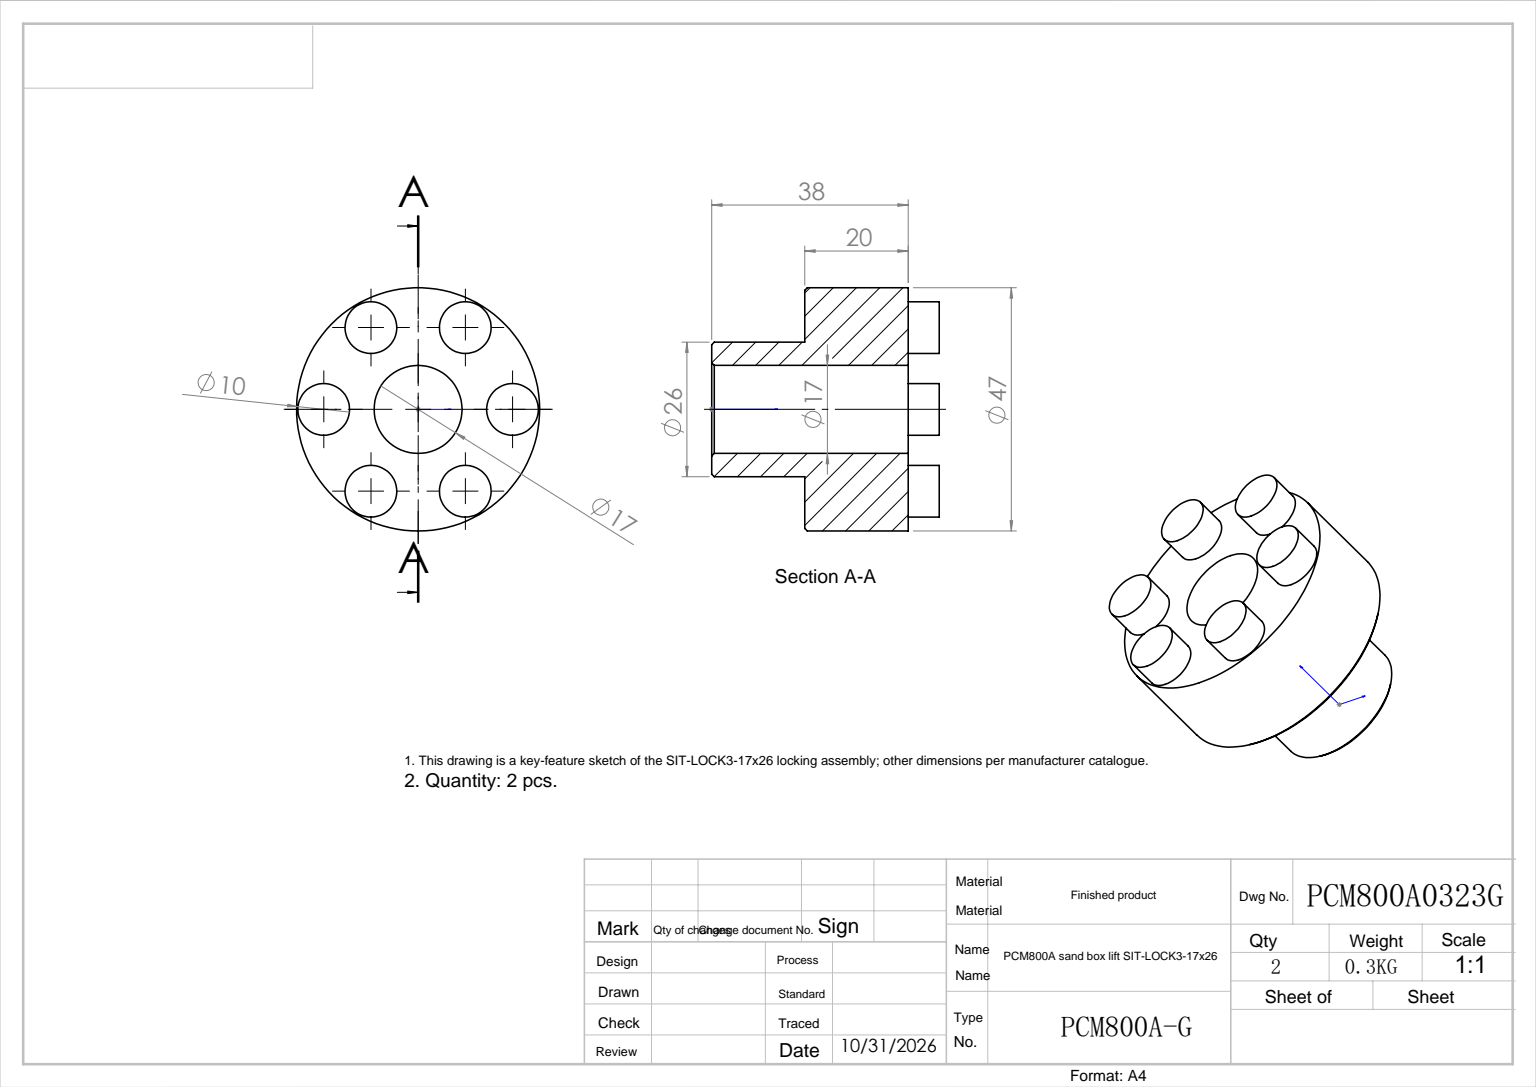
from build123d import *

# Parameters (mm, degrees)
SKETCH_1_R          = 13
SKETCH_1_R_2        = 8.5
EXTRUDE_1_DEPTH     = 18
SKETCH_2_R          = 23.5
EXTRUDE_2_DEPTH     = 20
SKETCH_3_R          = 8.5
CUT_EXTRUDE_1_DEPTH = 39.787884706
SKETCH_4_R          = 5
EXTRUDE_3_DEPTH     = 6
CHAMFER_1_SIZE      = 0.5


with BuildPart() as part:
    # 草图1 → 拉伸1 (new body)
    with BuildSketch(Plane(origin=(0, 0, 0), x_dir=(1, 0, 0), z_dir=(0, 1, 0))):
        with Locations(Location((0, 0, 0), (0, 0, 270))):
            Circle(SKETCH_1_R)
        with Locations(Location((0, 0, 0), (0, 0, 270))):
            Circle(SKETCH_1_R_2, mode=Mode.SUBTRACT)
    extrude(amount=EXTRUDE_1_DEPTH)

    # 草图2 → 拉伸2 (add)
    with BuildSketch(Plane(origin=(0, 18, 0), x_dir=(-1, 0, 0), z_dir=(0, 1, 0))):
        with Locations(Location((0, 0, 0), (0, 0, 90))):
            Circle(SKETCH_2_R)
    extrude(amount=EXTRUDE_2_DEPTH)

    # 草图3 → 切除-拉伸1 (cut, through all)
    with BuildSketch(Plane.XZ.offset(-18)):
        with Locations(Location((0, 0, 0), (0, 0, 270))):
            Circle(SKETCH_3_R)
    extrude(amount=-CUT_EXTRUDE_1_DEPTH, mode=Mode.SUBTRACT)

    # 草图4 → 拉伸3 (add)
    with BuildSketch(Plane(origin=(0, 38, 0), x_dir=(-1, 0, 0), z_dir=(0, 1, 0))):
        with Locations(Location((-18.25, 0, 0), (0, 0, 90))):
            Circle(SKETCH_4_R)
        with Locations(Location((-9.125, 15.804963619, 0), (0, 0, 90))):
            Circle(SKETCH_4_R)
        with Locations(Location((9.125, 15.804963619, 0), (0, 0, 90))):
            Circle(SKETCH_4_R)
        with Locations(Location((18.25, 0, 0), (0, 0, 90))):
            Circle(SKETCH_4_R)
        with Locations(Location((9.125, -15.804963619, 0), (0, 0, 90))):
            Circle(SKETCH_4_R)
        with Locations(Location((-9.125, -15.804963619, 0), (0, 0, 90))):
            Circle(SKETCH_4_R)
    extrude(amount=EXTRUDE_3_DEPTH)

    # 倒角1
    chamfer_1_edges = [part.edges().sort_by_distance(p)[0] for p in [
        (0, 0, -13),
        (0, 0, -8.5),
        (0, 18, -23.5),
    ]]
    chamfer(chamfer_1_edges, length=CHAMFER_1_SIZE)


solid = part.part
